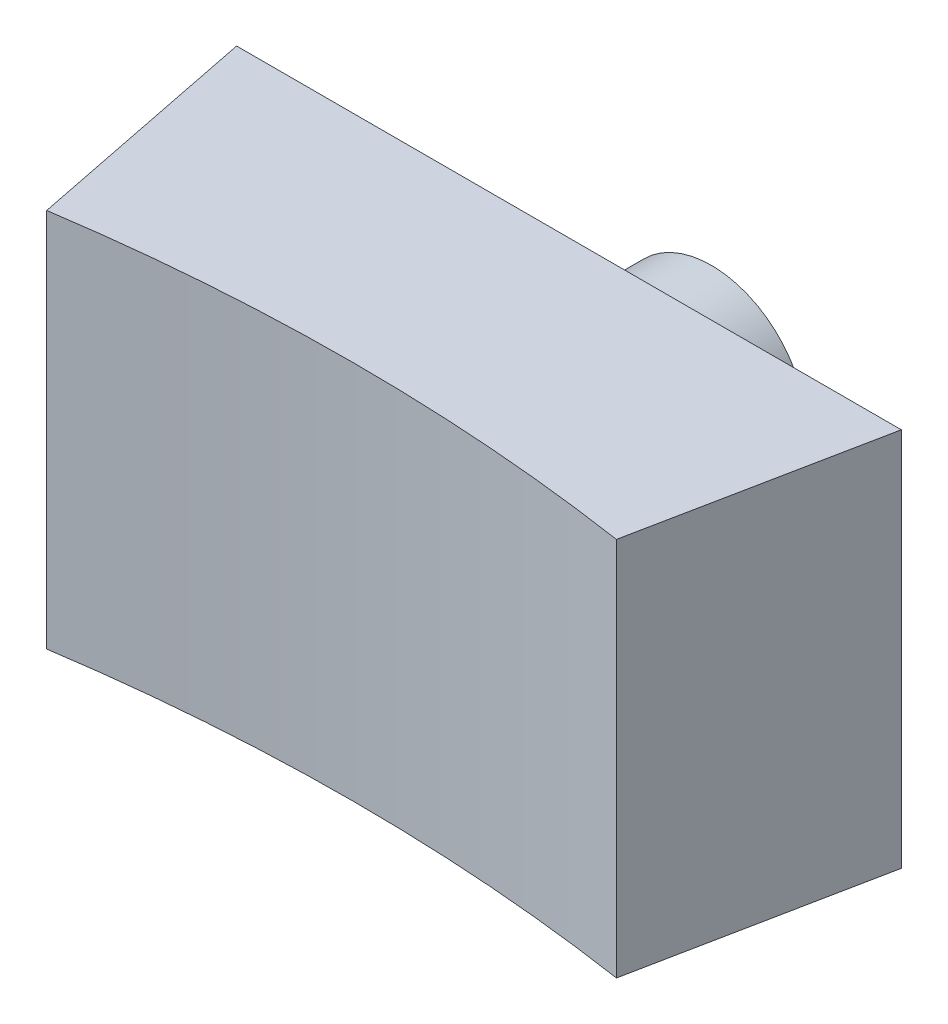
from build123d import *

# Parameters (mm, degrees)
BOSS_EXTRUDE1_DEPTH = 4
SKETCH2_R           = 2
SKETCH2_R_2         = 1.5
BOSS_EXTRUDE2_DEPTH = 3


with BuildPart() as part:
    # Sketch1 → Boss-Extrude1 (new, symmetric)
    with BuildSketch(Plane(origin=(0, 0, 0), x_dir=(1, 0, 0), z_dir=(0, 1, 0))):
        with BuildLine():
            Line((7, 0), (-7, 0))
            Line((-7, 0), (-6, -5))
            ThreePointArc((-6, -5), (0, -4.547439867), (6, -5))
            Line((6, -5), (7, 0))
        make_face()
    extrude(amount=BOSS_EXTRUDE1_DEPTH, both=True)

    # Sketch2 → Boss-Extrude2 (add)
    with BuildSketch(Plane.XY):
        Circle(SKETCH2_R)
        Circle(SKETCH2_R_2, mode=Mode.SUBTRACT)
    extrude(amount=-BOSS_EXTRUDE2_DEPTH)


solid = part.part
